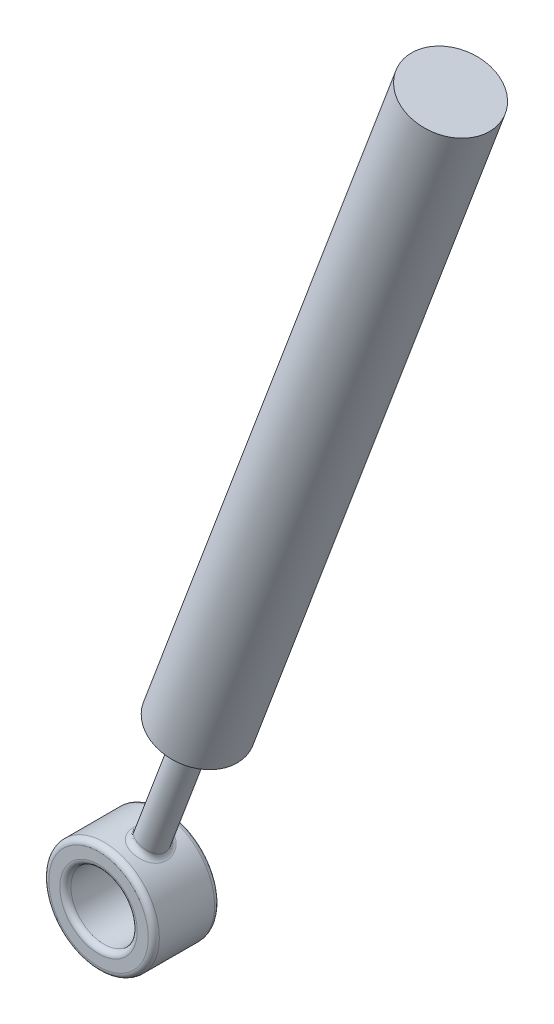
SolidWorks part; units mm, degrees
ref_plane "Front Plane" through (0, 0, 0) normal (0, 0, 1) x (1, 0, 0)
ref_plane "Top Plane" through (0, 0, 0) normal (0, 1, 0) x (1, 0, 0)
ref_plane "Right Plane" through (0, 0, 0) normal (1, 0, 0) x (0, 0, -1)
sketch "Sketch1" plane through (83.5733, 222.8927, 0) normal (-0.3511, -0.9363, 0) x (0.9363, -0.3511, 0)
  arc A0 (546.1928, 2320.0145) -> (546.1928, 2350.1259) centre (546.1928, 2335.0702) ccw construction
  arc A1 (546.1928, 2350.1259) -> (546.1928, 2320.0145) centre (546.1928, 2335.0702) ccw construction
  arc A2 (546.1928, 2320.0145) -> (546.1928, 2350.1259) centre (546.1928, 2335.0702) ccw
  arc A3 (546.1928, 2350.1259) -> (546.1928, 2320.0145) centre (546.1928, 2335.0702) ccw
extrude "Boss-Extrude1" add sketch "Sketch1" against normal up to surface (888.7199 mm away)
sketch "Sketch5" plane through (83.5733, 222.8927, 0) normal (-0.3511, -0.9363, 0) x (0.9363, -0.3511, 0)
  circle A0 centre (546.1928, 2335.0702) radius 5
  dimension "D1" = 10
sketch "Sketch6" plane through (0, 0, 2323.0702) normal (0, 0, -1) x (-1, 0, 0)
  arc A0 (-589.6761, -40.0266) -> (-552.2223, -25.9834) centre (-570.9492, -33.005) ccw construction
  arc A1 (-552.2223, -25.9834) -> (-589.6761, -40.0266) centre (-570.9492, -33.005) ccw construction
  arc A2 (-589.6761, -40.0266) -> (-552.2223, -25.9834) centre (-570.9492, -33.005) ccw
  arc A3 (-552.2223, -25.9834) -> (-589.6761, -40.0266) centre (-570.9492, -33.005) ccw
  arc A4 (-582.1853, -37.218) -> (-559.713, -28.792) centre (-570.9492, -33.005) ccw construction
  arc A5 (-559.713, -28.792) -> (-582.1853, -37.218) centre (-570.9492, -33.005) ccw construction
  arc A6 (-582.1853, -37.218) -> (-559.713, -28.792) centre (-570.9492, -33.005) ccw
  arc A7 (-559.713, -28.792) -> (-582.1853, -37.218) centre (-570.9492, -33.005) ccw
extrude "Boss-Extrude4" add sketch "Sketch6" against normal up to surface (24 mm away) separate body
extrude "Boss-Extrude5" add sketch "Sketch5" along normal up to surface (49.1351 mm away)
fillet "Fillet1" radius 2 1 edges at (582.3476, -16.571, 2334.091)
fillet "Fillet2" radius 2 4 edges at (582.9492, -33.005, 2347.0702) (558.9492, -33.005, 2323.0702) (550.9492, -33.005, 2323.0702) (590.9492, -33.005, 2347.0702)
chamfer "Chamfer2" distance 1 angle 45 1 edges at (599.68, 29.3792, 2335.0702)
